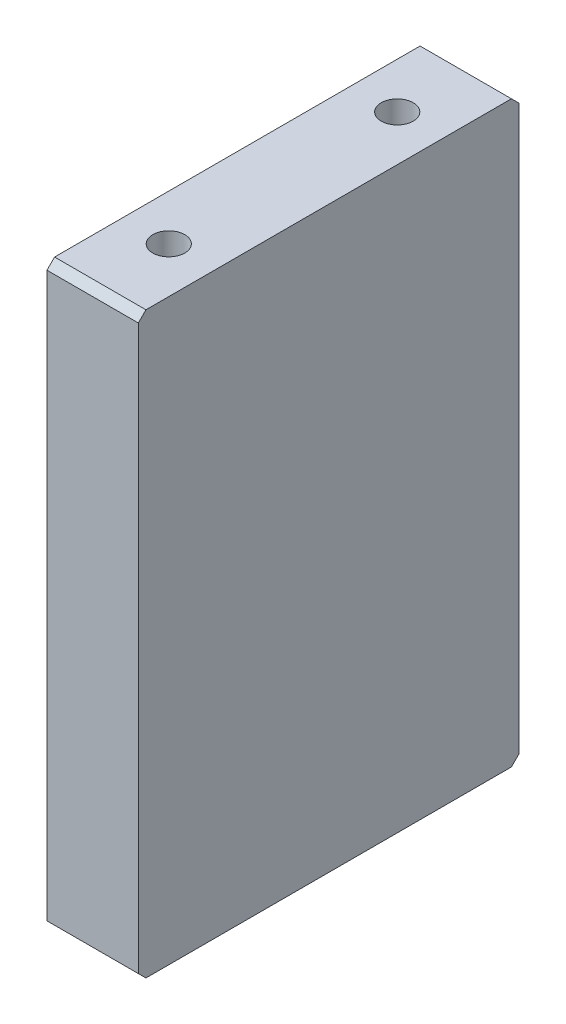
SolidWorks part; units mm, degrees
material "A7075"
ref_plane "Front Plane" through (0, 0, 0) normal (0, 0, 1) x (1, 0, 0)
ref_plane "Top Plane" through (0, 0, 0) normal (0, 1, 0) x (1, 0, 0)
ref_plane "Right Plane" through (0, 0, 0) normal (1, 0, 0) x (0, 0, -1)
sketch "Sketch6" plane through (0, 0, 0) normal (1, 0, 0) x (0, 0, -1)
  line L1 (0, 38) -> (50, 38)
  line L2 (0, 38) -> (0, -38)
  line L3 (0, -38) -> (50, -38)
  line L4 (50, 38) -> (50, -38)
  dimension "D1" = 76
  dimension "D2" = 50
extrude "Boss-Extrude6" add sketch "Sketch6" against normal blind 12 separate body
hole_wizard "M6 Tapped Hole2" positions "Sketch18" profile "Sketch17" tap size "M6" standard "Iso"
sketch "Sketch18" plane through (0, 0, 0) normal (1, 0, 0) x (0, 0, -1)
  line L1 (0, 38) -> (0, -38) construction
  point P0 (21, -30)
  point P2 (21, 30)
  dimension "D1" = 60
  dimension "D2" = 30
  dimension "D3" = 21
sketch "Sketch17" plane through (0, -30, -21) normal (0, 1, 0) x (0, 0, -1)
  line L0 (0, 0) -> (0, 16.5022)
  line L1 (0, 16.5022) -> (2.5, 15)
  line L2 (2.5, 15) -> (2.5, 0)
  line L5 (2.5, 0) -> (0, 0)
  line L10 (0, 16.5022) -> (-2.5, 15) construction
  line L11 (0, -6.35) -> (0, 107.95) construction
  dimension "螺纹孔钻头直径" = 5
  dimension "螺纹孔钻头深度" = 15
  dimension "导头角度" = 118
cosmetic thread "Cosmetic thread 10" [suppressed] parameters "D1"=12, "D2"=6
cosmetic thread "Cosmetic thread 11" [suppressed] parameters "D1"=12, "D2"=6
hole_wizard "M5 Tapped Hole3" positions "Sketch20" profile "Sketch19" tap size "M5" standard "Iso"
sketch "Sketch20" plane through (0, -38, 0) normal (0, -1, 0) x (-1, 0, 0)
  line L0 (12, 0) -> (0, 0) construction
  point P0 (6, 10)
  point P2 (6, 40)
  point P7 (6, 0)
  dimension "D1" = 10
  dimension "D2" = 30
sketch "Sketch19" plane through (-6, -38, -10) normal (1, 0, 0) x (0, 0, -1)
  line L0 (0, 0) -> (0, 18.6618)
  line L1 (0, 18.6618) -> (2.1, 17.4)
  line L2 (2.1, 17.4) -> (2.1, 0)
  line L5 (2.1, 0) -> (0, 0)
  line L10 (0, 18.6618) -> (-2.1, 17.4) construction
  line L11 (0, -6.35) -> (0, 107.95) construction
  dimension "螺纹孔钻头直径" = 4.2
  dimension "螺纹孔钻头深度" = 17.4
  dimension "导头角度" = 118
cosmetic thread "Cosmetic thread 25" parameters "D1"=15, "D2"=5
cosmetic thread "Cosmetic thread 26" parameters "D1"=15, "D2"=5
mirror "Mirror1" about plane through (0, 0, 0) normal (0, 1, 0) of "M5 Tapped Hole3"
hole_wizard "M5 Tapped Hole2" positions "Sketch22" profile "Sketch21" tap size "M5" standard "Iso"
sketch "Sketch22" plane through (0, 0, 0) normal (0, 0, 1) x (1, 0, 0)
  line L0 (-12, 38) -> (-12, -38) construction
  point P0 (-6, 15)
  point P2 (-6, -15)
  dimension "D1" = 30
  dimension "D2" = 15
  dimension "D3" = 6
sketch "Sketch21" plane through (-6, 15, 0) normal (1, 0, 0) x (0, -1, 0)
  line L0 (0, 0) -> (0, 13.6618)
  line L1 (0, 13.6618) -> (2.1, 12.4)
  line L2 (2.1, 12.4) -> (2.1, 0)
  line L5 (2.1, 0) -> (0, 0)
  line L10 (0, 13.6618) -> (-2.1, 12.4) construction
  line L11 (0, -6.35) -> (0, 107.95) construction
  dimension "螺纹孔钻头直径" = 4.2
  dimension "螺纹孔钻头深度" = 12.4
  dimension "导头角度" = 118
cosmetic thread "Cosmetic thread 27" [suppressed] parameters "D1"=10, "D2"=5
cosmetic thread "Cosmetic thread 28" [suppressed] parameters "D1"=10, "D2"=5
chamfer "Chamfer1" distance 1 angle 45 4 edges at (-6, 38, 0) (-6, 38, -50) (-6, -38, -50) (-6, -38, 0)
